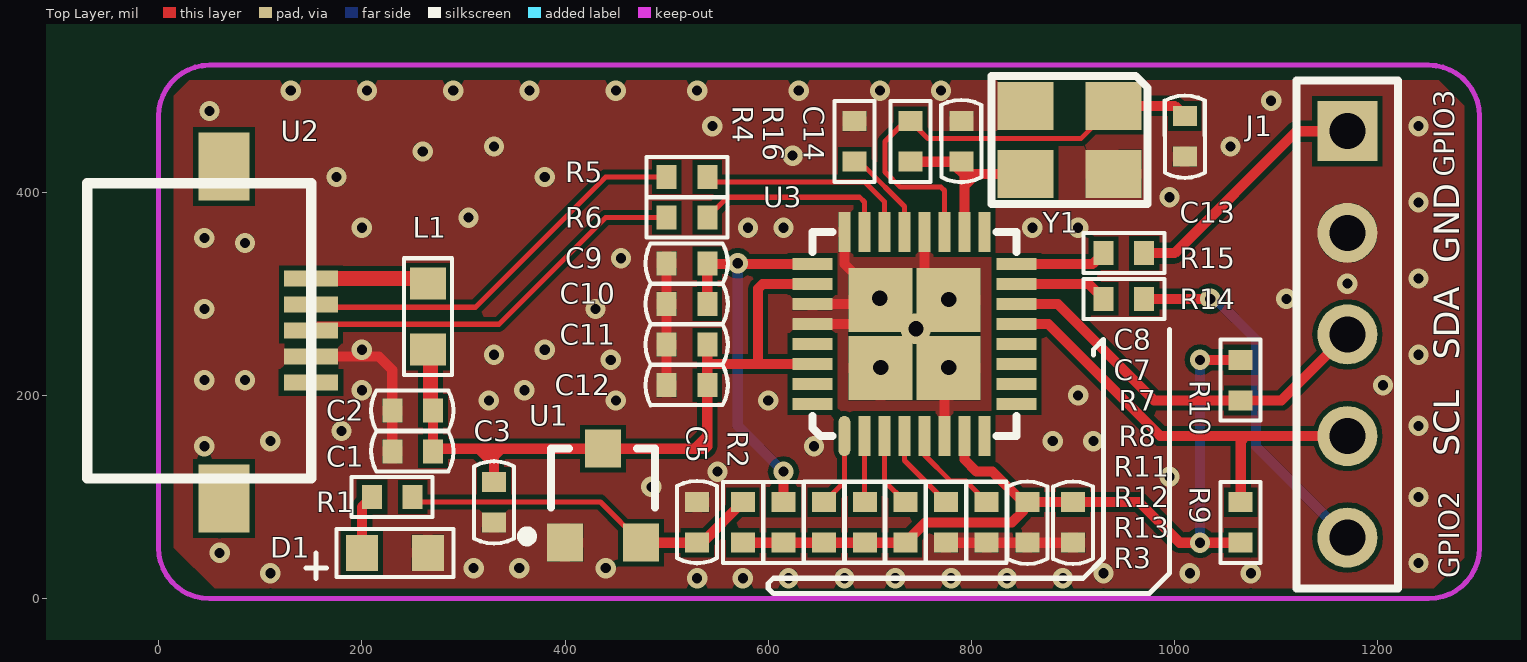
[diagram p0: Top Layer view]
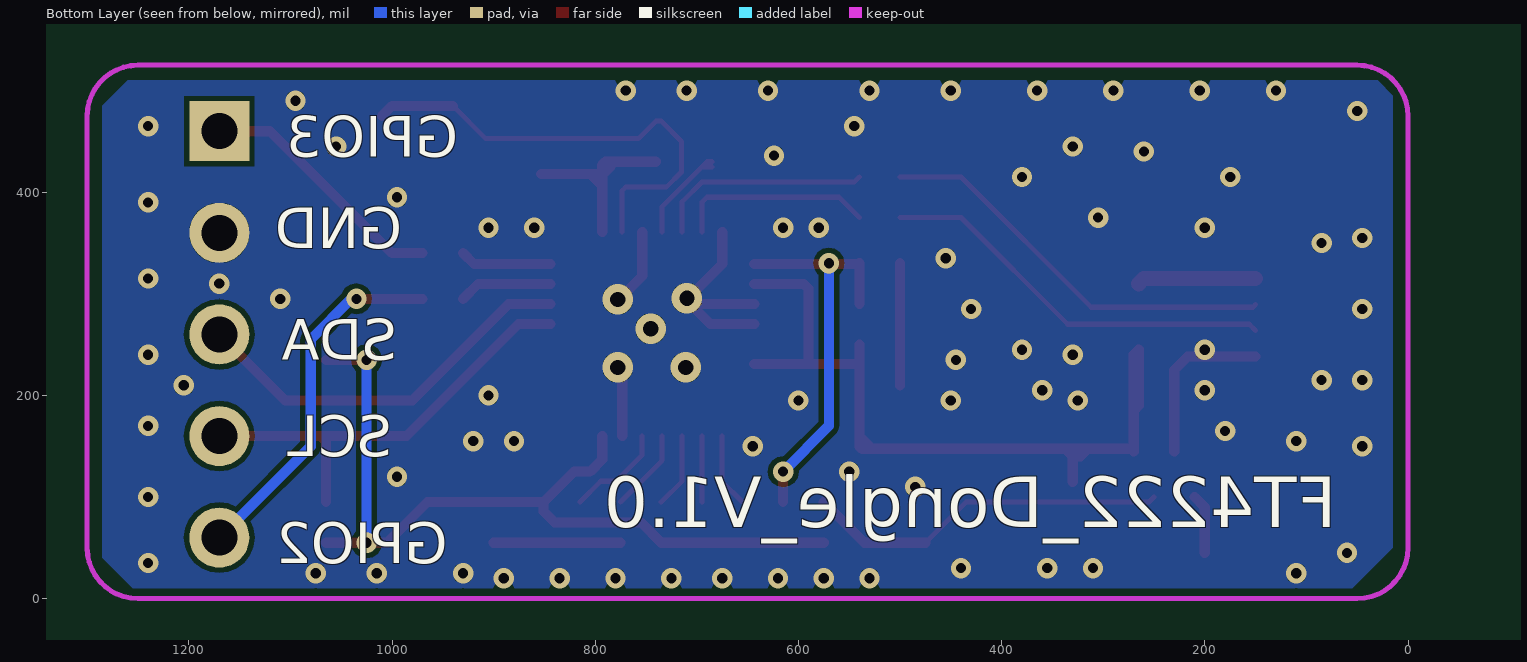
[diagram p1: Bottom Layer view, seen from below]
# Altium PCB MISC82699.PcbDoc
Units mil, origin at the board's own origin, x right, y up, seen from the top; angles counter-clockwise.
Board outline 6000 x 4000 mil, 2 copper layers (Top Layer, Bottom Layer); 35 components, 25 nets, 115 pads, 87 vias.

## Layer stack, top to bottom (the 12.6 mil dielectric is the usual default, probably not edited)
Top Solder: solder mask 0.4, Solder Resist, Dk 3.5
Top Layer: signal copper 1.4
Dielectric 1: dielectric 12.6, FR-4, Dk 4.8
Bottom Layer: signal copper 1.4
Bottom Solder: solder mask 0.4, Solder Resist, Dk 3.5

## Board outline
-2050,-1830 3950,-1830 3950,2170 -2050,2170

## Design rules (kind name [scope] priority, off if disabled: settings)
AssemblyTestPointUsage [All] p1 off:
AssemblyTestpoint [All] p1 off: testpointundercomponent=TRUE minsize=40 maxsize=100 preferedsize=60 minholesize=0 maxholesize=40 preferedholesize=32 testpointgrid=1 usegrid=TRUE gridtolerance=0.01 allowsidetop=TRUE allowsidebottom=TRUE
Clearance [All] p1: gap=5
ComponentClearance [All] p1 off: gap=0 collisioncheckmode=3 verticalgap=0 showdistances=FALSE
DiffPairsRouting [All] p1 off: maxlimit=10 minlimit=10 mostfreqgap=10 toplayer_minwidth=15 toplayer_maxwidth=15 toplayer_prefwidth=15 bottomlayer_minwidth=15 bottomlayer_maxwidth=15 bottomlayer_prefwidth=15 maxuncoupledlength=500
FabricationTestPointUsage [All] p1 off: valid=0 allowmultiple=FALSE
FabricationTestpoint [All] p1 off: side=3 testpointundercomponent=TRUE minsize=40 maxsize=100 preferedsize=60 minholesize=0 maxholesize=40 preferedholesize=32 testpointgrid=1 allowsidetop=TRUE allowsidebottom=TRUE usegrid=TRUE gridtolerance=0.01
FanoutControl Fanout_BGA [IsBGA] p1 off: bgadir=Out bgaviamode=Centered fanoutstyle=Auto fanoutdirection=Alternating viagrid=1 // Fanout_BGA (Default Rule)
FanoutControl Fanout_LCC [IsLCC] p2 off: bgadir=Out bgaviamode=Centered fanoutstyle=Auto fanoutdirection=Alternating viagrid=1 // Fanout_LCC (Default Rule)
FanoutControl Fanout_SOIC [IsSOIC] p3 off: bgadir=Out bgaviamode=Centered fanoutstyle=Auto fanoutdirection=Alternating viagrid=1 // Fanout_SOIC (Default Rule)
FanoutControl Fanout_Small [(CompPinCount < 5)] p4 off: bgadir=Out bgaviamode=Centered fanoutstyle=Auto fanoutdirection=OutThenIn viagrid=1 // Fanout_Small (Default Rule)
FanoutControl Fanout_Default [All] p5 off: bgadir=Out bgaviamode=Centered fanoutstyle=Auto fanoutdirection=Alternating viagrid=1 // Fanout_Default (Default Rule)
Height [All] p1 off: minheight=0 maxheight=1000 prefheight=500
HoleSize [All] p1 off: absolutevalues=TRUE maxlimit=100 minlimit=1 maxpercent=80.000 minpercent=20.000
HoleToHoleClearance [All] p1 off: gap=10 allowstackedmicrovias=TRUE
LayerPairs [All] p1 off: enforce=TRUE
MinimumSolderMaskSliver [All] p1 off: minsoldermaskwidth=10
NetAntennae [All] p1 off: netantennaetolerance=0
PasteMaskExpansion [All] p1 off: expansion=0
PlaneClearance [All] p1 off: clearance=5
PlaneConnect [All] p1 off: planeconnectstyle=Direct reliefexpansion=20 reliefentries=4 reliefconductorwidth=10 reliefairgap=10
PolygonConnect [All] p1 off: connectstyle=Direct reliefconductorwidth=10 reliefentries=4 polygonreliefangle="90 Angle" airgapwidth=10
RoutingCorners [All] p1 off: cornerstyle=45-Degree minsetback=100 maxsetback=100
RoutingLayers [All] p1 off: top layer_v5=TRUE bottom layer_v5=TRUE
RoutingPriority [All] p1 off: routingpriority=0
RoutingTopology [All] p1 off: topology=Shortest
RoutingVias [All] p1: holewidth=10 width=20 viastyle="Through Hole" minholewidth=5 minwidth=5 maxholewidth=30 maxwidth=50
SilkToBoardRegionClearance [All] p1 off:
SilkToSilkClearance [All] p1 off: silktosilkclearance=0
SilkToSolderMaskClearance [IsPad] p1 off: minsilkscreentomaskgap=0 clearancetoexposedcopper=TRUE
SolderMaskExpansion [All] p1 off: expansion=4
Width [All] p1: maxlimit=50 minlimit=5 preferedwidth=10
2 further rules are at their usual default settings.

## Components (designator, comment, footprint, x,y, rotation, side; value= is the part's Value field where it differs from the comment)
C1 "4.7uF" C0402 230,145 r0 top
C2 "0.1uF" C0402 230,185 r0 top
C3 "4.7uF" C0402 330,75 r90 top
C5 "4.7uF" C0402 530,95 r270 top
C7 "4.7uF" C0402 855,55 r90 top
C8 "0.1uF" C0402 900,55 r90 top
C9 "4.7uF" C0402 500,330 r0 top
C10 "0.1uF" C0402 500,290 r0 top
C11 "4.7uF" C0402 500,250 r0 top
C12 "0.1uF" C0402 500,210 r0 top
C13 "20pF" C0402 1010,435 r90 top
C14 "20pF" C0402 790,470 r270 top
D1 "Led" R0603 265,45 r180 top
J1 "PIN 2.54*5" DIP2.54*5 1170,460 r270 top
L1 "000R" R0603 265,245 r90 top
R1 "470ohm" R0402 250,100 r180 top
R2 "000R" R0402 575,95 r270 top
R3 "NC" R0402 615,95 r270 top
R4 "12K" R0402 685,470 r270 top
R5 "000R" R0402 500,415 r0 top
R6 "000R" R0402 500,375 r0 top
R7 "000R" R0402 815,55 r90 top
R8 "000R" R0402 775,55 r90 top
R9 "1K" R0402 1065,95 r270 top
R10 "1K" R0402 1065,195 r90 top
R11 "10K" R0402 735,55 r90 top
R12 "10K" R0402 695,55 r90 top
R13 "10K" R0402 655,55 r90 top
R14 "000R" R0402 930,295 r0 top
R15 "000R" R0402 930,340 r0 top
R16 "1M" R0402 740,470 r270 top
U1 "AX6601" SOT_23 400,55 r0 top
U2 "USB" MicroUSB 150,315 r270 top locked
U3 "FT4222" QFN32 675,160 r90 top
Y1 "12M" XTAL_3225 940,485 r180 top

## Footprints (in the part's own frame and the unit in brackets; to place one, negate y for a bottom-side part, rotate by r counter-clockwise, add the part's x,y. Pads: shape width x height; smd on the part's side, far side on the other; paste and mask are expansions set on the pad)
C0402 [mm]
  rect 0.5x0.6 smd: 1(0,0) 2(1.016,0)
  silkscreen extent -0.53,-0.5 1.53,0.5
DIP2.54*5 [mm]
  rect 1.5x1.5 hole 0.9: 1(0,0)
  round 1.5 hole 0.9: 2(2.54,0) 3(5.08,0) 4(7.62,0)
  round 1.499 hole 0.899: 5(10.16,0)
  silkscreen extent -1.27,-1.27 11.43,1.27
MicroUSB [mm]
  rect 1.7x1.28 smd: 0(-2.8,-2.178) 0(5.5,-2.178)
  rect 0.4x1.35 smd: 1(0,0) 2(0.65,0) 3(1.3,0) 4(1.95,0) 5(2.6,0)
  silkscreen extent -2.38,-5.6 5,0
QFN32 [mm]
  oval 1x0.3 smd: 1(0,0)
  rect 1x0.3 smd: 2(0,-0.5) 3(0,-1) 4(0,-1.5) 5(0,-2) 6(0,-2.5) 7(0,-3) 8(0,-3.5) 17(5.1,-3.5) 18(5.1,-3) 19(5.1,-2.5) 20(5.1,-2) 21(5.1,-1.5) 22(5.1,-1) 23(5.1,-0.5) 24(5.1,0)
  rect 0.3x1 smd: 9(0.8,-4.3) 10(1.3,-4.3) 11(1.8,-4.3) 12(2.3,-4.3) 13(2.8,-4.3) 14(3.3,-4.3) 15(3.8,-4.3) 16(4.3,-4.3) 25(4.3,0.8) 26(3.8,0.8) 27(3.3,0.8) 28(2.8,0.8) 29(2.3,0.8) 30(1.8,0.8) 31(1.3,0.8) 32(0.8,0.8)
  rect 1.6x1.6 smd: 33(1.7,-2.6) 33(1.7,-0.9) 33(3.4,-2.6) 33(3.4,-0.9)
  silkscreen extent 0,-4.3 5.1,0.8
R0402 [mm]
  rect 0.5x0.6 smd: 1(0,0) 2(1.016,0)
  silkscreen extent -0.5,-0.5 1.52,0.5
R0603 [mm]
  rect 0.8x0.9 smd: 1(0,0) 2(1.651,0)
  silkscreen extent -0.64,-0.6 2.29,0.6
SOT_23 [mm]
  rect 0.9x0.95 smd: 1(0,0) 2(1.9,0) 3(0.95,2.35)
  silkscreen extent -1.08,0.03 2.25,2.35
XTAL_3225 [mm]
  rect 1.4x1.2 smd: 1(0,0) 2(2.2,0) 3(2.2,1.7) 4(0,1.7)
  silkscreen extent -0.85,-0.75 3.05,2.46

## Part data
C1 C2 C3 C5 C7 C8 C9 C10 C11 C12 C13 C14: library part Cap
J1: library part PIN_5
L1: library part Inductor
R1 R2 R3 R4 R5 R6 R7 R8 R9 R10 R11 R12 R13 R14 R15 R16: library part Res
U1: library part LDO
U2: library part "Micro USB"
Y1: library part Crystal

## Via types
v1: diameter 20, hole 10, Top Layer to Bottom Layer, 82 vias
v2: diameter 30, hole 15, Top Layer to Bottom Layer, 5 vias

## Nets (pads, with @x,y where several pads share a name; then routed paths per layer and width w, separated by ;. In a path a pad name is that pad's centre, name@x,y a point inside that pad or via, vN(x,y) a via of type N, cw(c..) or ccw(c..) an arc to the next point about the centre after c; other vN are vias at no path point)
DM: R5.1 U2.2 | length 404.2
  Top Layer w5: U2.2 152.66,286.75 311.75,286.75 440,415 R5.1
DP: R6.1 U2.3 | length 396.1
  Top Layer w5: U2.3 156.18,270 335,270 440,375 R6.1
GND: C1.1 C2.1 C3.1 C5.1 C7.1 C8.1 C9.1 C10.1 C11.1 C12.1 C13.1 C14.1 D1.1 J1.2 R4.1 R7.1 R8.1 U1.1 U2.4 U3.6 U3.20 U3.24 U3.27 U3.28 U3.33 Y1.2 Y1.4 | length 777.1
  Top Layer w10: U2.4 216.77,238.23 230,225 C2.1 C1.1 ; C12.1 C11.1 C10.1 C9.1 ; U3.28 686.81,270.24 U3.33@706.5,289.92 ; U3.27 U3.33@706.5,289.92 ; U3.24 675,329.29 710.43,293.86 U3.33@706.5,289.92 ; U3.20 753.74,317.48 U3.33@777.36,293.86 ; U3.6 773.43,222.99 U3.33@777.36,226.93 ; R8.1 R7.1 C7.1 C8.1
  other v1: 530,20 575,20 620,20 675,20 725,20 780,20 835,20 890,20 110,25 930,25 1015,25 1075,25 310,30 355,30 440,30 1240,35 60,45 1240,100 485,110 995,120 550,125 45,150 645,150 110,155 880,155 920,155 180,165 1240,170 325,195 450,195 600,195 905,200 200,205 360,205 1205,210 45,215 85,215 445,235 330,240 1240,240 200,245 380,245 45,285 430,285 1110,295 1170,310 1240,315 455,335 85,350 45,355 200,365 580,365 615,365 860,365 905,365 305,375 1240,390 995,395 175,415 380,415 623.99,436.02 260,440 330,445 1055,445 545,465 1240,465 50,480 1095,490 130,500 205,500 290,500 365,500 450,500 530,500 630,500 710,500 770,500
  other v2: 710.81,227.49 777.74,227.49 745.38,265.56 777.74,294.41 709.67,295.56
GPIO2: J1.5 R14.2 | length 358.8
  Top Layer w10: R14.2 v1(1035,295)
  Bottom Layer w10: v1(1035,295) 1040,295 1080,255 1080,150 J1.5
GPIO3: J1.1 R15.2 | length 249.7
  Top Layer w10: R15.2 1000,340 1120,460 J1.1
LDO1V8: C5.2 R1.1 R2.1 U1.2 | length 360.2
  Top Layer w5: R1.1 255,95 434.8,95 U1.2
  Top Layer w10: U1.2 C5.2 535,55 R2.1
NetC13_2: C13.2 R16.1 U3.19 Y1.1 | length 464.9
  Top Layer w5: U3.19 773.43,401.57 770,405 730,405 715,420 715,450 735,470 R16.1 757.34,452.66 907.66,452.66 Y1.1
  Top Layer w10: Y1.1 1000,485 C13.2
NetC14_2: C14.2 R16.2 U3.18 Y1.3 | length 217.4
  Top Layer w10: R16.2 C14.2 ; U3.18 793.11,406.18 ; Y1.3 805,418.07 ; C14.2 793.11,426.89 793.11,416.89 ; C14.2 785,425 793.11,416.89 ; 793.11,406.18 793.11,415 ; 793.11,406.18 805,418.07 ; 793.11,415 796.18,418.07 805,418.07 ; 793.11,415 793.11,416.89
NetD1_2: D1.2 R1.2 | length 59.1
  Top Layer w10: D1.2 200,90 R1.2
NetL1_2: L1.2 U2.1 | length 117.1
  Top Layer w15: U2.1 260,315 L1.2
NetR4_2: R4.2 U3.21 | length 102.5
  Top Layer w5: R4.2@685,425 R4.2@695,425 ; R4.2 690,430 R4.2@695,425 ; U3.21 734.05,385.95 R4.2@695,425
NetR5_2: R5.2 U3.22 | length 214.3
  Top Layer w5: R5.2 545,410 695,410 714.37,390.63 U3.22
NetR6_2: R6.2 U3.23 | length 194.4
  Top Layer w5: R6.2 560,395 690,395 694.68,390.32 U3.23
NetR7_2: R7.2 U3.5 | length 99.2
  Top Layer w5: U3.5 753.74,141.26 779.53,115.47 794.53,115.47 R7.2
NetR8_2: R8.2 U3.4 | length 82
  Top Layer w5: U3.4 734.05,135.95 R8.2
NetR11_2: R11.2 U3.3 | length 73.5
  Top Layer w5: U3.3 714.37,115.63 R11.2
NetR12_2: R12.2 U3.2 | length 65.1
  Top Layer w5: U3.2 694.68,95.32 R12.2
NetR13_2: R13.2 U3.1 | length 73.3
  Top Layer w5: R13.2 675,115 U3.1
NetR14_1: R14.1 U3.15 | length 91.8
  Top Layer w10: U3.15 915.39,309.61 R14.1
NetR15_1: R15.1 U3.16 | length 90.1
  Top Layer w10: U3.16 919.29,329.29 R15.1
SCL: J1.4 R9.1 U3.13 | length 438.4
  Top Layer w10: U3.13 875.56,270.24 985.8,160 1070,160 ; R9.1 1065,155 1070,160 ; J1.4 1070,160
SDA: J1.3 R10.1 U3.14 | length 392
  Top Layer w10: U3.14 885.08,289.92 980,195 R10.1 1105,195 J1.3
VCC3V3: C9.2 C10.2 R3.1 U3.25 | length 397.4
  Top Layer w10: C10.2 C9.2 540.71,329.29 U3.25 ; R3.1 v1(615,125)
  Bottom Layer w10: v1(570,330) 570,170 v1(615,125)
VCCIO: C7.2 C8.2 R2.2 R3.2 R9.2 R10.2 R11.1 R12.1 R13.1 U3.7 | length 846.7
  Top Layer w10: R2.2 R3.2 R13.1 R12.1 R11.1 755,75 840,75 850.8,85.8 C7.2@850.8,95 ; U3.7 793.11,136.89 805,125 820.8,125 C7.2@850.8,95 ; v1(1025,235) R10.2 ; R9.2 v1(1025,55) 1005,55 965,95 C8.2 C7.2 C7.2@850.8,95
  Bottom Layer w10: v1(1025,55) v1(1025,235)
VIN: C1.2 C2.2 C3.2 C11.2 C12.2 L1.1 U1.3 U3.26 U3.30 | length 841.9
  Top Layer w10: C3.2 330,140 ; C11.2 540,230 ; U3.30 592.18,230.87 ; U3.26 594.61,309.61 590,305 590,233.05 592.18,230.87 ; C2.2 265,190 L1.1 270,240 C2.2 ; C2.2 C1.2 272.52,147.52 315,147.52 ; 315,147.52 322.52,140 330,140 ; 315,147.52 337.52,147.52 ; 330,140 337.52,147.52 ; 337.52,147.52 U1.3 527.52,147.52 ; 527.52,147.52 540,160 ; 527.52,147.52 537.52,147.52 540,150 540,160 ; 540,160 C12.2 540,230 ; 540,230 540.87,230.87 592.18,230.87
pads on no net: U2.0 U2.5 U3.8 U3.9 U3.10 U3.11 U3.12 U3.17 U3.29 U3.31 U3.32

## Polygon pours and split planes (outlines as drawn)
GND on Bottom Layer "GND Layer-No Net" (solid, remove dead copper, pour order 11): 15,495 30,510 1260,510 1285,485 1285,40 1255,10 55,10 15,50 15,495
GND on Top Layer "GND Layer-No Net" (solid, remove dead copper, pour order 7): 15,495 30,510 35,510 1260,510 1280,490 1285,485 1285,40 1260,15 1255,10 1250,10 55,10 15,50 15,495

## Keep-outs
Keep-Out Layer:
  lines w5: 0,475 cw(c50,475) 50,525 1250,525 cw(c1250,475) 1300,475 1300,50.79 ; 0,476.26 0,50 ccw(c50,50) 50,0 1250,0 ccw(c1250,50) 1300,50

## Silkscreen, mask and mechanical layers (free items; w line width, h text height)
Top Overlay:
  lines w5: 145,30 165,30 ; 155,20 155,45 ; 920,240 920,245 930,255 930,40 910,20 605,20 600,15 600,10 605,5 975,5 995,25 995,265
  text "GPIO3" at 1275,415 h20 r90
  text "GND" at 1280,330 h25 r90
  text "SDA" at 1280,235 h25 r90
  text "SCL" at 1280,140 h25 r90
  text "GPIO2" at 1280,20 h20 r90
Bottom Overlay:
  text "GPIO3" at 935,435 h40
  text "GND" at 990,345 h40
  text "SDA" at 995,235 h40
  text "SCL" at 1000,140 h40
  text "FT4222_Dongle_V1.0" at 70,70 h50
  text "GPIO2" at 945,35 h40